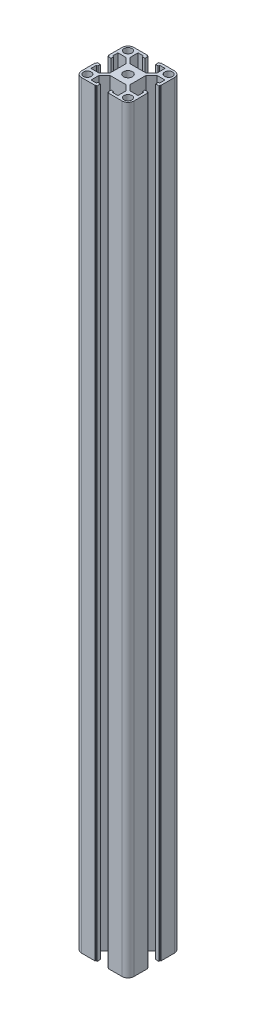
from build123d import *

# Parameters (mm, degrees)
SKETCH16_R     = 3.4
SKETCH16_R_2   = 3
MEMBER_1_DEPTH = 580


with BuildPart() as part:
    # Sketch16 → Member 1 (new body)
    with BuildSketch(Plane(origin=(0, 0, 0), x_dir=(-1, 0, 0), z_dir=(0, 1, 0))):
        with BuildLine():
            Line((-5.1, 20), (-5.1, 19.5))
            Line((-5.1, 19.5), (-4.1, 19.5))
            Line((-4.1, 19.5), (-4.1, 17))
            Line((-4.1, 17), (-6.1, 17))
            Line((-6.1, 17), (-6.1, 18))
            Line((-6.1, 18), (-10.3, 18))
            Line((-10.3, 18), (-10.3, 12))
            Line((-10.3, 12), (-6, 7.7))
            Line((-6, 7.7), (6, 7.7))
            Line((6, 7.7), (10.3, 12))
            Line((10.3, 12), (10.3, 18))
            Line((10.3, 18), (6.1, 18))
            Line((6.1, 18), (6.1, 17))
            Line((6.1, 17), (4.1, 17))
            Line((4.1, 17), (4.1, 19.5))
            Line((4.1, 19.5), (5.1, 19.5))
            Line((5.1, 19.5), (5.1, 20))
            Line((5.1, 20), (15.5, 20))
            ThreePointArc((15.5, 20), (18.681980515, 18.681980515), (20, 15.5))
            Line((20, 15.5), (20, 5.1))
            Line((20, 5.1), (19.5, 5.1))
            Line((19.5, 5.1), (19.5, 4.1))
            Line((19.5, 4.1), (17, 4.1))
            Line((17, 4.1), (17, 6.1))
            Line((17, 6.1), (18, 6.1))
            Line((18, 6.1), (18, 10.3))
            Line((18, 10.3), (12, 10.3))
            Line((12, 10.3), (7.7, 6))
            Line((7.7, 6), (7.7, -6))
            Line((7.7, -6), (12, -10.3))
            Line((12, -10.3), (18, -10.3))
            Line((18, -10.3), (18, -6.1))
            Line((18, -6.1), (17, -6.1))
            Line((17, -6.1), (17, -4.1))
            Line((17, -4.1), (19.5, -4.1))
            Line((19.5, -4.1), (19.5, -5.1))
            Line((19.5, -5.1), (20, -5.1))
            Line((20, -5.1), (20, -15.5))
            ThreePointArc((20, -15.5), (18.681980515, -18.681980515), (15.5, -20))
            Line((15.5, -20), (5.1, -20))
            Line((5.1, -20), (5.1, -19.5))
            Line((5.1, -19.5), (4.1, -19.5))
            Line((4.1, -19.5), (4.1, -17))
            Line((4.1, -17), (6.1, -17))
            Line((6.1, -17), (6.1, -18))
            Line((6.1, -18), (10.3, -18))
            Line((10.3, -18), (10.3, -12))
            Line((10.3, -12), (6, -7.7))
            Line((6, -7.7), (-6, -7.7))
            Line((-6, -7.7), (-10.3, -12))
            Line((-10.3, -12), (-10.3, -18))
            Line((-10.3, -18), (-6.1, -18))
            Line((-6.1, -18), (-6.1, -17))
            Line((-6.1, -17), (-4.1, -17))
            Line((-4.1, -17), (-4.1, -19.5))
            Line((-4.1, -19.5), (-5.1, -19.5))
            Line((-5.1, -19.5), (-5.1, -20))
            Line((-5.1, -20), (-15.5, -20))
            ThreePointArc((-15.5, -20), (-18.681980515, -18.681980515), (-20, -15.5))
            Line((-20, -15.5), (-20, -5.1))
            Line((-20, -5.1), (-19.5, -5.1))
            Line((-19.5, -5.1), (-19.5, -4.1))
            Line((-19.5, -4.1), (-17, -4.1))
            Line((-17, -4.1), (-17, -6.1))
            Line((-17, -6.1), (-18, -6.1))
            Line((-18, -6.1), (-18, -10.3))
            Line((-18, -10.3), (-12, -10.3))
            Line((-12, -10.3), (-7.7, -6))
            Line((-7.7, -6), (-7.7, 6))
            Line((-7.7, 6), (-12, 10.3))
            Line((-12, 10.3), (-18, 10.3))
            Line((-18, 10.3), (-18, 6.1))
            Line((-18, 6.1), (-17, 6.1))
            Line((-17, 6.1), (-17, 4.1))
            Line((-17, 4.1), (-19.5, 4.1))
            Line((-19.5, 4.1), (-19.5, 5.1))
            Line((-19.5, 5.1), (-20, 5.1))
            Line((-20, 5.1), (-20, 15.5))
            ThreePointArc((-20, 15.5), (-18.681980515, 18.681980515), (-15.5, 20))
            Line((-15.5, 20), (-5.1, 20))
        make_face()
        Circle(SKETCH16_R, mode=Mode.SUBTRACT)
        with Locations((-15.556349186, 15.556349186)):
            Circle(SKETCH16_R_2, mode=Mode.SUBTRACT)
        with Locations((15.556349186, 15.556349186)):
            Circle(SKETCH16_R_2, mode=Mode.SUBTRACT)
        with Locations((15.556349186, -15.556349186)):
            Circle(SKETCH16_R_2, mode=Mode.SUBTRACT)
        with Locations((-15.556349186, -15.556349186)):
            Circle(SKETCH16_R_2, mode=Mode.SUBTRACT)
    extrude(amount=MEMBER_1_DEPTH)


solid = part.part
